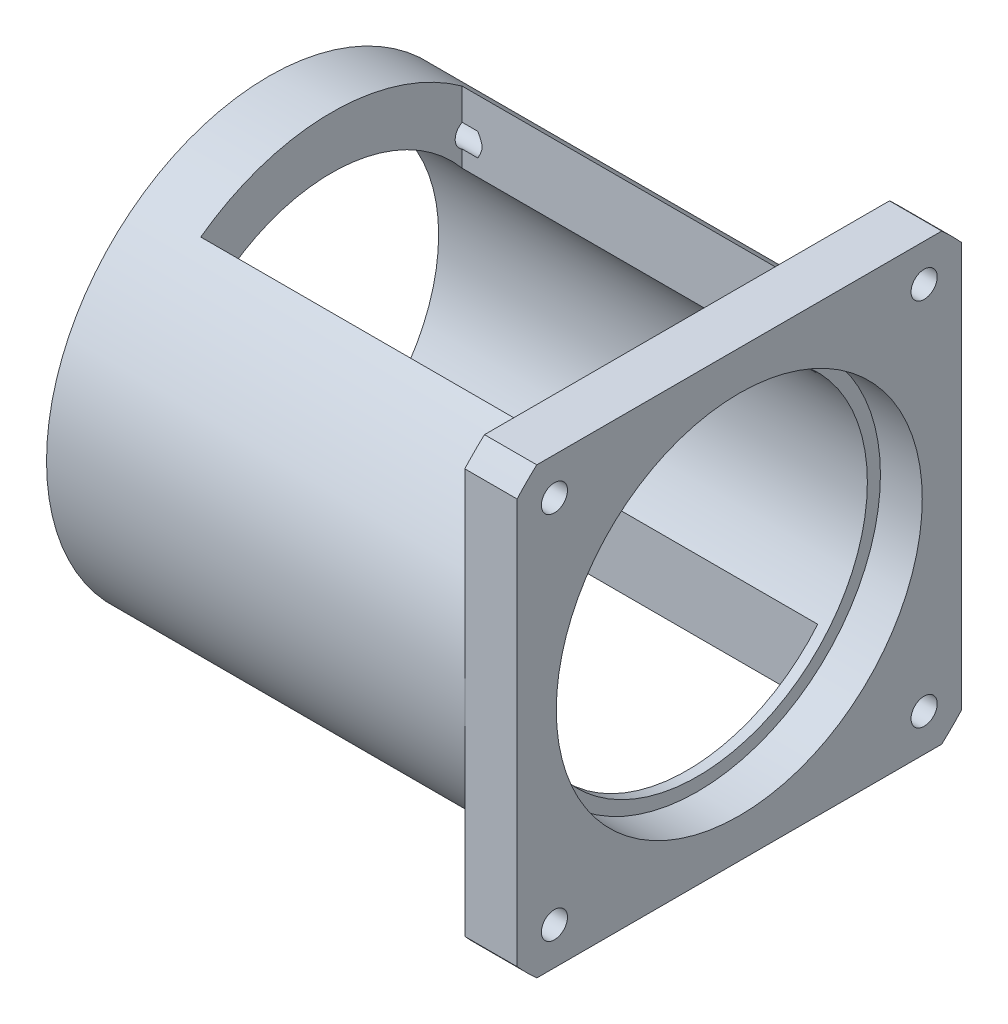
from build123d import *

# Parameters (mm, degrees)
SKETCH_1_R               = 42.5
EXTRUDE_1_DEPTH          = 80
SKETCH_2_R               = 57.5
EXTRUDE_2_DEPTH          = 10
SKETCH_3_OUTSIDE_W       = 154.176
SKETCH_3_OUTSIDE_H       = 154.176
SKETCH_3_OUTSIDE_W_2     = 85
SKETCH_3_OUTSIDE_H_2     = 85
CUT_EXTRUDE_1_DEPTH      = 122.295094707
SKETCH_4_R               = 35
CUT_EXTRUDE_2_DEPTH      = 8
PATTERN_CIRCULAR_1_COUNT = 4
SKETCH_7_R               = 32.5
CUT_EXTRUDE_3_DEPTH      = 102.668579217
CUT_EXTRUDE_4_DEPTH      = 109.22430411
CUT_EXTRUDE_4_DEPTH_BACK = 109.22430411
SKETCH_8_W               = 68
SKETCH_8_H               = 50
PATTERN_CIRCULAR_2_COUNT = 4


with BuildPart() as part:
    # 草图1 → 凸台-拉伸1 (new body)
    with BuildSketch(Plane(origin=(0, 0, 0), x_dir=(0, 0, -1), z_dir=(1, 0, 0))):
        Circle(SKETCH_1_R)
    extrude(amount=EXTRUDE_1_DEPTH)

    # 草图2 → 凸台-拉伸2 (add)
    with BuildSketch(Plane(origin=(80, 0, 0), x_dir=(0, 0, -1), z_dir=(1, 0, 0))):
        Circle(SKETCH_2_R)
    extrude(amount=EXTRUDE_2_DEPTH)

    # 草图3 outside → 切除-拉伸1 (cut, through all)
    with BuildSketch(Plane(origin=(90, 0, 0), x_dir=(0, 0, -1), z_dir=(1, 0, 0))):
        Rectangle(SKETCH_3_OUTSIDE_W, SKETCH_3_OUTSIDE_H)
        Rectangle(SKETCH_3_OUTSIDE_W_2, SKETCH_3_OUTSIDE_H_2, mode=Mode.SUBTRACT)
    extrude(amount=-CUT_EXTRUDE_1_DEPTH, mode=Mode.SUBTRACT)

    # 草图4 → 切除-拉伸2 (cut)
    with BuildSketch(Plane(origin=(90, 0, 0), x_dir=(0, 0, -1), z_dir=(1, 0, 0))):
        Circle(SKETCH_4_R)
    extrude(amount=-CUT_EXTRUDE_2_DEPTH, mode=Mode.SUBTRACT)

    # 草图6 → M6 螺纹孔1 (revolve, cut)
    with BuildSketch(Plane(origin=(90, 35.355339059, 35.355339059), x_dir=(0, 0, -1), z_dir=(0, 1, 0))):
        Polygon((0, 0), (0, 16.502151548), (2.5, 15), (2.5, 0), align=None)
    hole_wizard_m6_1 = revolve(axis=Axis((96.35, 35.355339059, 35.355339059), (-1, 0, 0)), mode=Mode.SUBTRACT)

    # 阵列(圆周)1: M6 螺纹孔1 ×4 about axis
    pattern_circular_1_axis = Axis((0, 0, 0), (1, 0, 0))
    for i in range(1, PATTERN_CIRCULAR_1_COUNT):
        add(hole_wizard_m6_1.rotate(pattern_circular_1_axis, i * 360 / PATTERN_CIRCULAR_1_COUNT), mode=Mode.SUBTRACT)

    # 草图7 → 切除-拉伸3 (cut, through all)
    with BuildSketch(Plane(origin=(82, 0, 0), x_dir=(0, 0, -1), z_dir=(1, 0, 0))):
        Circle(SKETCH_7_R)
    extrude(amount=-CUT_EXTRUDE_3_DEPTH, mode=Mode.SUBTRACT)

    # 草图8 → 切除-拉伸4 (cut, two sides: drawn at the far end of the back side and taken through both)
    with BuildSketch(Plane(origin=(0, 0, 0), x_dir=(1, 0, 0), z_dir=(0, 1, 0)).offset(-CUT_EXTRUDE_4_DEPTH_BACK)):
        with Locations((46, 0)):
            Rectangle(SKETCH_8_W, SKETCH_8_H)
    extrude(amount=CUT_EXTRUDE_4_DEPTH + CUT_EXTRUDE_4_DEPTH_BACK, mode=Mode.SUBTRACT)

    # 草图10 → M6 螺纹孔2 (revolve, cut)
    with BuildSketch(Plane(origin=(0, 26.162950904, -26.162950904), x_dir=(0, 0, 1), z_dir=(0, 1, 0))):
        Polygon((0, 0), (0, 16.502151548), (2.5, 15), (2.5, 0), align=None)
    hole_wizard_m6_2 = revolve(axis=Axis((-6.35, 26.162950904, -26.162950904), (1, 0, 0)), mode=Mode.SUBTRACT)

    # 阵列(圆周)2: M6 螺纹孔2 ×4 about axis
    pattern_circular_2_axis = Axis((0, 0, 0), (1, 0, 0))
    for i in range(1, PATTERN_CIRCULAR_2_COUNT):
        add(hole_wizard_m6_2.rotate(pattern_circular_2_axis, i * 360 / PATTERN_CIRCULAR_2_COUNT), mode=Mode.SUBTRACT)


solid = part.part
